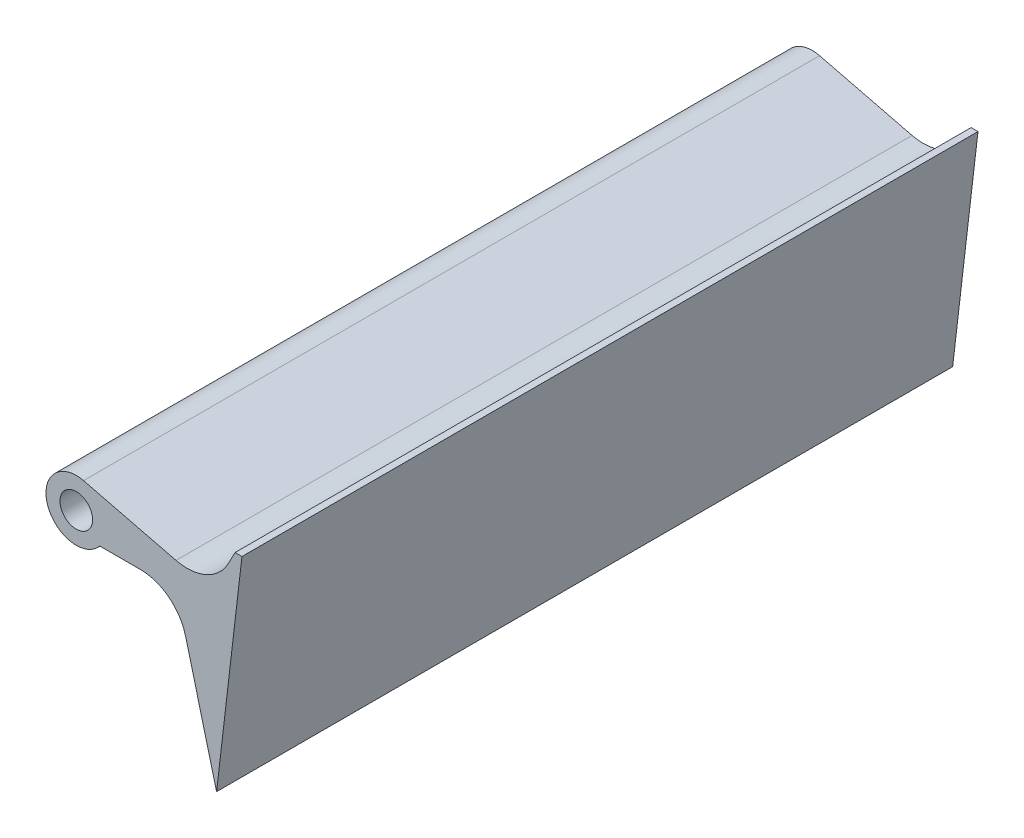
SolidWorks part; units mm, degrees
ref_plane "Front Plane" through (0, 0, 0) normal (0, 0, 1) x (1, 0, 0)
ref_plane "Top Plane" through (0, 0, 0) normal (0, 1, 0) x (1, 0, 0)
ref_plane "Right Plane" through (0, 0, 0) normal (1, 0, 0) x (0, 0, -1)
sketch "Sketch1" plane through (0, 0, 0) normal (0, 0, 1) x (1, 0, 0)
  line L0 (7.7913, 31.5523) -> (145.2584, -2.393)
  line L1 (145.2584, -2.393) -> (170.4123, 46.0283)
  line L2 (107.4339, -20.5387) -> (150.6228, -186.1304)
  line L3 (150.6228, -186.1304) -> (177.8183, 46.0283)
  line L4 (107.4339, -20.5387) -> (25.1875, -20.5387)
  line L5 (177.8183, 46.0283) -> (170.4123, 46.0283)
  arc A0 (7.7913, 31.5523) -> (25.1875, -20.5387) centre (0, 0) ccw
  circle A1 centre (0, 0) radius 17.5
  dimension "D1" = 65
  dimension "D2" = 35
extrude "Boss-Extrude1" add sketch "Sketch1" along normal blind 790
fillet "Fillet1" radius 50 1 edges at (145.2584, -2.393, 395)
fillet "Fillet3" radius 50 1 edges at (107.4339, -20.5387, 395)
